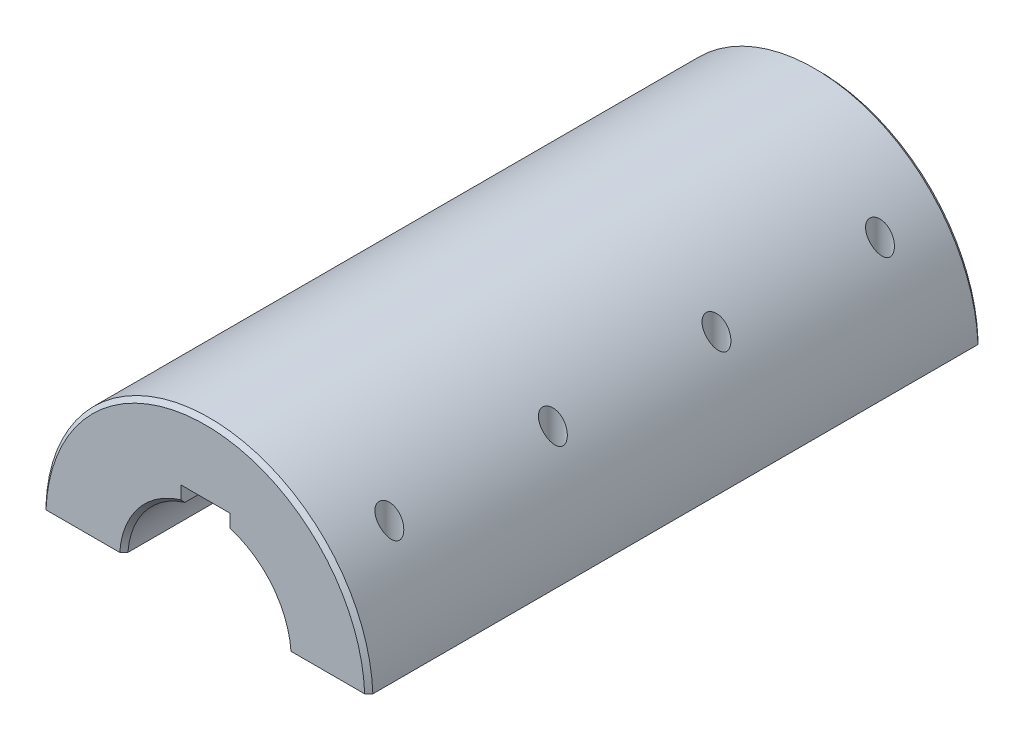
SolidWorks part; units mm, degrees
material "Plain carbon steel"
ref_plane "Front Plane" through (0, 0, 0) normal (0, 0, 1) x (1, 0, 0)
ref_plane "Top Plane" through (0, 0, 0) normal (0, 1, 0) x (1, 0, 0)
ref_plane "Right Plane" through (0, 0, 0) normal (1, 0, 0) x (0, 0, -1)
sketch "Sketch1" plane through (0, 0, 0) normal (0, 0, 1) x (1, 0, 0)
  line L0 (0, 23.3) -> (0, 0) construction
  line L1 (-6, 23.3) -> (6, 23.3)
  line L2 (-6, 23.3) -> (-6, 19.0788)
  line L4 (6, 23.3) -> (6, 19.0788)
  arc A0 (-6, 19.0788) -> (6, 19.0788) centre (0, 0) ccw
  circle A1 centre (0, 0) radius 40
  dimension "D1" = 40
  dimension "D2" = 80
  dimension "D4" = 23.3
  dimension "D3" = 12
extrude "Boss-Extrude1" add sketch "Sketch1" along normal mid plane 150
chamfer "Chamfer1" distance 1 angle 45 4 edges at (0, -20, 75) (40, 0, 75) (0, -20, -75) (40, 0, -75)
sketch "Sketch2" plane through (0, 0, 75) normal (0, 0, 1) x (1, 0, 0)
  line L1 (-41, 1.5) -> (41, 1.5)
  line L2 (-41, 1.5) -> (-41, -1.5)
  line L3 (-41, -1.5) -> (41, -1.5)
  line L4 (41, 1.5) -> (41, -1.5)
  line L5 (-41, 1.5) -> (41, -1.5) construction
  line L6 (-41, -1.5) -> (41, 1.5) construction
  point P0 (0, 0)
  dimension "D1" = 3
  dimension "D2" = 82
extrude "Cut-Extrude1" cut sketch "Sketch2" against normal blind 170
hole_wizard "M6 Tapped Hole1" positions "Sketch4" profile "Sketch5" tap size "M6" standard "GB"
sketch "Sketch4" plane through (0, 1.5, 0) normal (0, -1, 0) x (-1, 0, 0)
  point P0 (-30, -60)
  dimension "D1" = 60
  dimension "D2" = 30
sketch "Sketch5" plane through (30, 1.5, 60) normal (1, 0, 0) x (0, 0, -1)
  line L0 (0, 0) -> (0, 40.5022)
  line L1 (0, 40.5022) -> (2.5, 39)
  line L2 (2.5, 39) -> (2.5, 0)
  line L5 (2.5, 0) -> (0, 0)
  line L10 (0, 40.5022) -> (-2.5, 39) construction
  line L11 (0, -6.35) -> (0, 107.95) construction
  dimension "螺纹孔钻头直径" = 5
  dimension "螺纹孔钻头深度" = 39
  dimension "导头角度" = 118
cosmetic thread "Hole thread1" parameters "D1"=36, "D2"=6
pattern_linear "LPattern1" count 4 spacing 40 along (0, 0, -1) count 2 spacing 60 along (-1, 0, 0) of "M6 Tapped Hole1"
cosmetic thread "Hole thread2" parameters "D1"=36, "D2"=6
cosmetic thread "Hole thread3" parameters "D1"=36, "D2"=6
cosmetic thread "Hole thread4" parameters "D1"=36, "D2"=6
cosmetic thread "Hole thread5" parameters "D1"=36, "D2"=6
cosmetic thread "Hole thread6" parameters "D1"=36, "D2"=6
cosmetic thread "Hole thread7" parameters "D1"=36, "D2"=6
cosmetic thread "Hole thread8" parameters "D1"=36, "D2"=6
